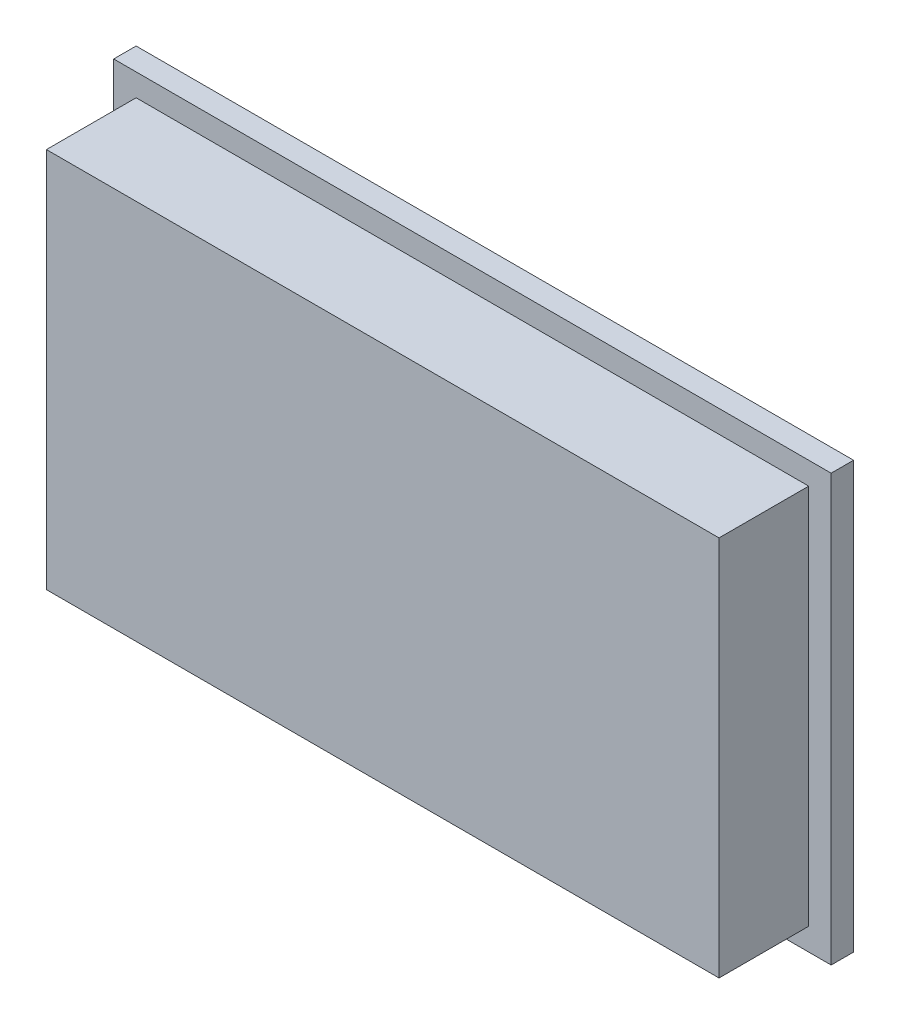
from build123d import *

# Parameters (mm, degrees)
SKETCH_1_W      = 64
SKETCH_1_H      = 38
EXTRUDE_1_DEPTH = 1
SKETCH_2_W      = 60
SKETCH_2_H      = 34
EXTRUDE_2_DEPTH = 9


with BuildPart() as part:
    # 草图1 → 凸台-拉伸1 (new, symmetric)
    with BuildSketch(Plane.XY):
        Rectangle(SKETCH_1_W, SKETCH_1_H)
    extrude(amount=EXTRUDE_1_DEPTH, both=True)

    # 草图2 → 凸台-拉伸2 (add)
    with BuildSketch(Plane.XY):
        Rectangle(SKETCH_2_W, SKETCH_2_H)
    extrude(amount=EXTRUDE_2_DEPTH)


solid = part.part
